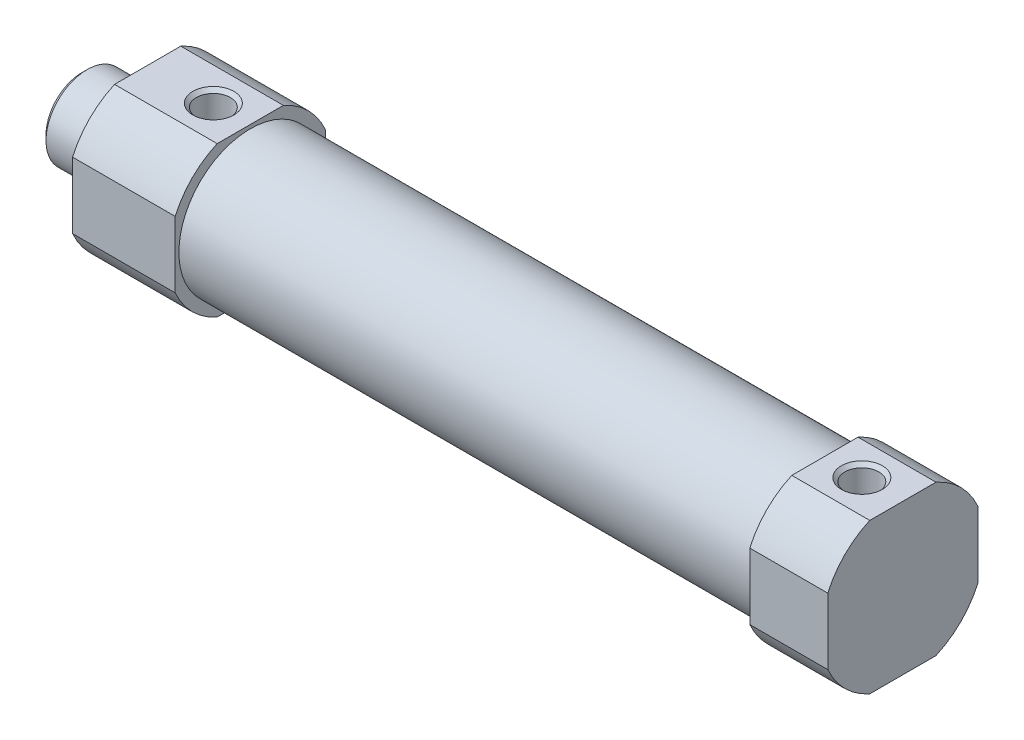
from build123d import *

# Parameters (mm, degrees)
BOSS_EXTRUDE1_DEPTH = 12.5
SKETCH3_R           = 8.7
BOSS_EXTRUDE2_DEPTH = 70
BOSS_EXTRUDE3_DEPTH = 9.5
HOLE1_D             = 4.134
HOLE1_DEPTH         = 5.5
HOLE1_CSINK_D       = 5
HOLE1_CSINK_ANGLE   = 90
HOLE1_TIP           = 1.193383006
HOLE2_D             = 4.134
HOLE2_DEPTH         = 5.5
HOLE2_CSINK_D       = 5
HOLE2_CSINK_ANGLE   = 90
HOLE2_TIP           = 1.193383006


with BuildPart() as part:
    # Sketch1 → Revolve1 (revolve)
    with BuildSketch(Plane.XY, mode=Mode.PRIVATE) as revolve1_sk:
        Polygon((-8, 0), (-8, 4.3865), (-7.3865, 5), (0, 5), (0, 0), align=None)
    revolve(revolve1_sk.sketch.rotate(Axis((0, 0, 0), (-1, 0, 0)), 270), axis=Axis((0, 0, 0), (-1, 0, 0)))

    # Sketch2 → Boss-Extrude1 (add)
    with BuildSketch(Plane(origin=(0, 0, 0), x_dir=(0, 0, -1), z_dir=(1, 0, 0))):
        with BuildLine():
            Line((-4.034538387, -9.15), (4.034538387, -9.15))
            ThreePointArc((4.034538387, -9.15), (7.071067812, -7.071067812), (9.15, -4.034538387))
            Line((9.15, -4.034538387), (9.15, 4.034538387))
            ThreePointArc((9.15, 4.034538387), (7.071067812, 7.071067812), (4.034538387, 9.15))
            Line((4.034538387, 9.15), (-4.034538387, 9.15))
            ThreePointArc((-4.034538387, 9.15), (-7.071067812, 7.071067812), (-9.15, 4.034538387))
            Line((-9.15, 4.034538387), (-9.15, -4.034538387))
            ThreePointArc((-9.15, -4.034538387), (-7.071067812, -7.071067812), (-4.034538387, -9.15))
        make_face()
    extrude(amount=BOSS_EXTRUDE1_DEPTH)

    # Sketch3 → Boss-Extrude2 (add)
    with BuildSketch(Plane(origin=(12.5, 0, 0), x_dir=(0, 0, -1), z_dir=(1, 0, 0))):
        Circle(SKETCH3_R)
    extrude(amount=BOSS_EXTRUDE2_DEPTH)

    # Sketch4 → Boss-Extrude3 (add)
    with BuildSketch(Plane(origin=(82.5, 0, 0), x_dir=(0, 0, -1), z_dir=(1, 0, 0))):
        with BuildLine():
            Line((-4.034538387, -9.15), (4.034538387, -9.15))
            ThreePointArc((4.034538387, -9.15), (7.071067812, -7.071067812), (9.15, -4.034538387))
            Line((9.15, -4.034538387), (9.15, 4.034538387))
            ThreePointArc((9.15, 4.034538387), (7.071067812, 7.071067812), (4.034538387, 9.15))
            Line((4.034538387, 9.15), (-4.034538387, 9.15))
            ThreePointArc((-4.034538387, 9.15), (-7.071067812, 7.071067812), (-9.15, 4.034538387))
            Line((-9.15, 4.034538387), (-9.15, -4.034538387))
            ThreePointArc((-9.15, -4.034538387), (-7.071067812, -7.071067812), (-4.034538387, -9.15))
        make_face()
    extrude(amount=BOSS_EXTRUDE3_DEPTH)

    # Hole1
    with Locations(Plane(origin=(0, 9.15, 0), x_dir=(1, 0, 0), z_dir=(0, 1, 0))):
        with Locations((8, 0)):
            CounterSinkHole(HOLE1_D / 2, HOLE1_CSINK_D / 2, depth=HOLE1_DEPTH, counter_sink_angle=HOLE1_CSINK_ANGLE)
            with Locations((0, 0, -(HOLE1_DEPTH + HOLE1_TIP / 2))):  # 120° drill point
                Cone(0, HOLE1_D / 2, HOLE1_TIP, mode=Mode.SUBTRACT)

    # Hole2
    with Locations(Plane(origin=(0, 9.15, 0), x_dir=(1, 0, 0), z_dir=(0, 1, 0))):
        with Locations((87, 0)):
            CounterSinkHole(HOLE2_D / 2, HOLE2_CSINK_D / 2, depth=HOLE2_DEPTH, counter_sink_angle=HOLE2_CSINK_ANGLE)
            with Locations((0, 0, -(HOLE2_DEPTH + HOLE2_TIP / 2))):  # 120° drill point
                Cone(0, HOLE2_D / 2, HOLE2_TIP, mode=Mode.SUBTRACT)

    # Sketch9 → Cut-Revolve1 (revolve, cut)
    with BuildSketch(Plane.XY, mode=Mode.PRIVATE) as cut_revolve1_sk:
        Polygon((-8, 0), (-8, 2.5), (12.5, 2.5), (12.5, 8), (62.5, 8), (62.5, 0), align=None)
    revolve(cut_revolve1_sk.sketch.rotate(Axis((50, 0, 0), (-1, 0, 0)), 270), axis=Axis((50, 0, 0), (-1, 0, 0)), mode=Mode.SUBTRACT)


solid = part.part
